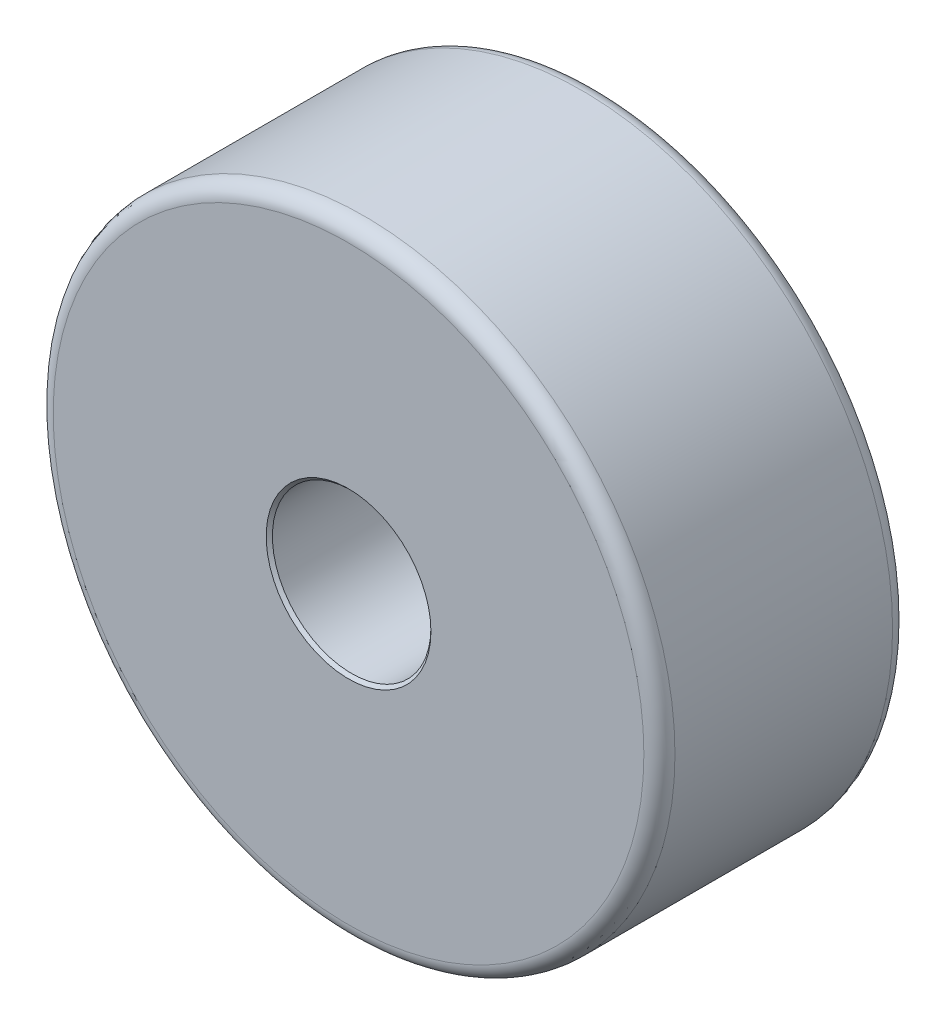
SolidWorks part; units mm, degrees
material "45"
ref_plane "Front Plane" through (0, 0, 0) normal (0, 0, 1) x (1, 0, 0)
ref_plane "Top Plane" through (0, 0, 0) normal (0, 1, 0) x (1, 0, 0)
ref_plane "Right Plane" through (0, 0, 0) normal (1, 0, 0) x (0, 0, -1)
sketch "Sketch1" plane through (0, 0, 0) normal (0, 0, 1) x (1, 0, 0)
  circle A0 centre (0, 0) radius 100
  circle A1 centre (0, 0) radius 25.5
  dimension "D1" = 200
  dimension "D2" = 51
extrude "Boss-Extrude1" add sketch "Sketch1" along normal blind 80
fillet "Fillet1" radius 5 2 edges at (100, 0, 0) (100, 0, 80)
chamfer "Chamfer1" distance 1 angle 45 2 edges at (25.5, 0, 80) (25.5, 0, 0)
